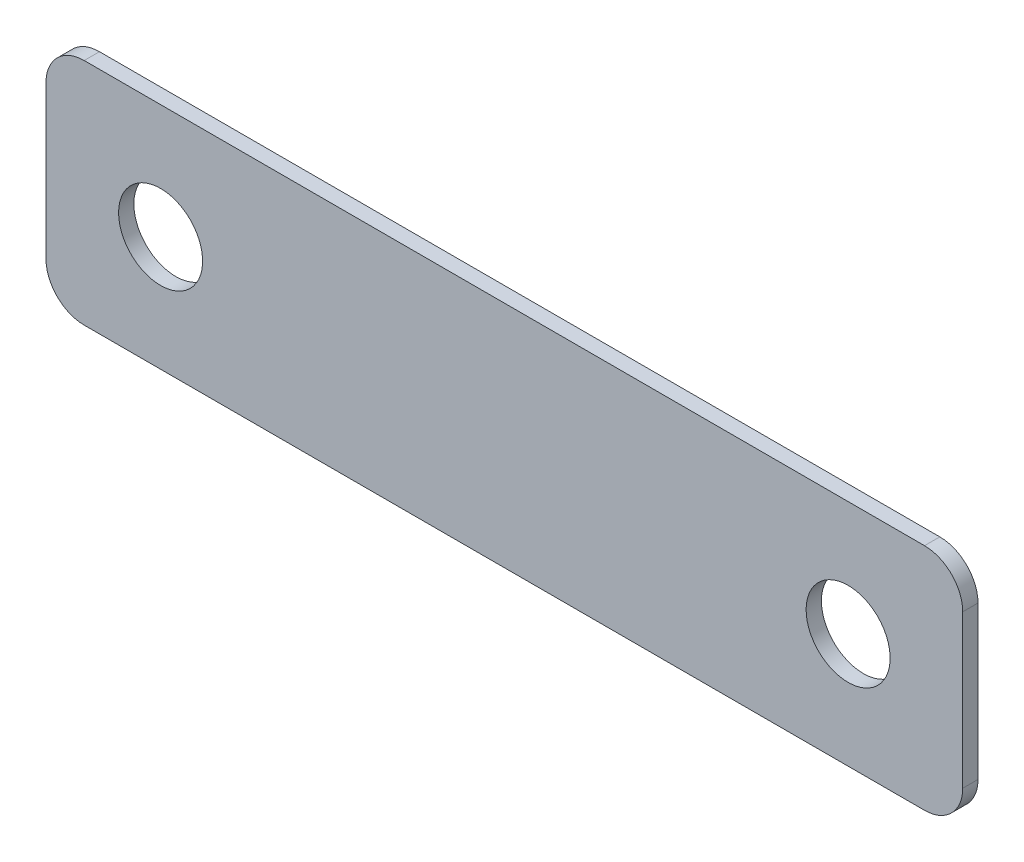
from build123d import *

# Parameters (mm, degrees)
SKETCH_1_W          = 120
SKETCH_1_H          = 30
EXTRUDE_1_DEPTH     = 2
SKETCH_2_R          = 5.5
CUT_EXTRUDE_1_DEPTH = 10
FILLET_1_R          = 5


with BuildPart() as part:
    # 草图1 → 凸台-拉伸1 (new body)
    with BuildSketch(Plane.XY):
        Rectangle(SKETCH_1_W, SKETCH_1_H)
    extrude(amount=EXTRUDE_1_DEPTH)

    # 草图2 → 切除-拉伸1 (cut)
    with BuildSketch(Plane(origin=(0, 0, 0), x_dir=(-1, 0, 0), z_dir=(0, 0, -1))):
        with Locations((45, 0)):
            Circle(SKETCH_2_R)
        with Locations((-45, 0)):
            Circle(SKETCH_2_R)
    extrude(amount=-CUT_EXTRUDE_1_DEPTH, mode=Mode.SUBTRACT)

    # 圆角1
    fillet_1_edges = [part.edges().sort_by_distance(p)[0] for p in [
        (60, -15, 1),
        (-60, -15, 1),
        (-60, 15, 1),
        (60, 15, 1),
    ]]
    fillet(fillet_1_edges, radius=FILLET_1_R)


solid = part.part
